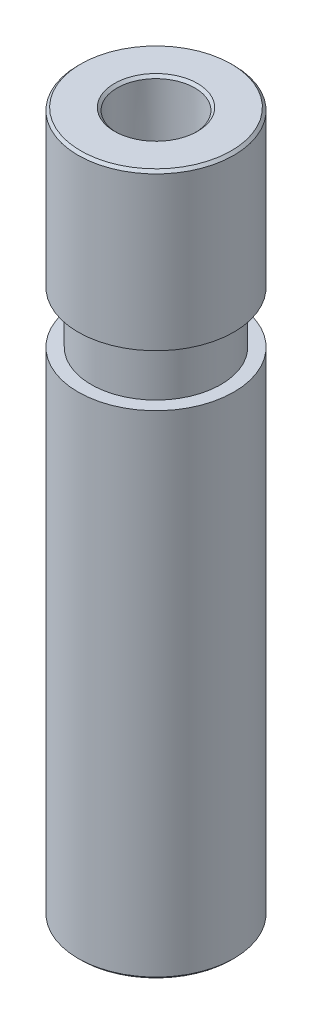
from build123d import *


with BuildPart() as part:
    # Sketch1 → Revolve1 (revolve)
    with BuildSketch(Plane.XY, mode=Mode.PRIVATE) as revolve1_sk:
        Polygon((1.1, 0), (2.9, 0), (3, 0.1), (3, 19), (2.5, 19), (2.5, 21), (3, 21), (3, 26.9), (2.9, 27), (1.6, 27), (1.498148466, 26.900017142), (1.001851534, 0.099982858), align=None)
    revolve(revolve1_sk.sketch.rotate(Axis((0, 0, 0), (0, 1, 0)), 90), axis=Axis((0, 0, 0), (0, 1, 0)))


solid = part.part
